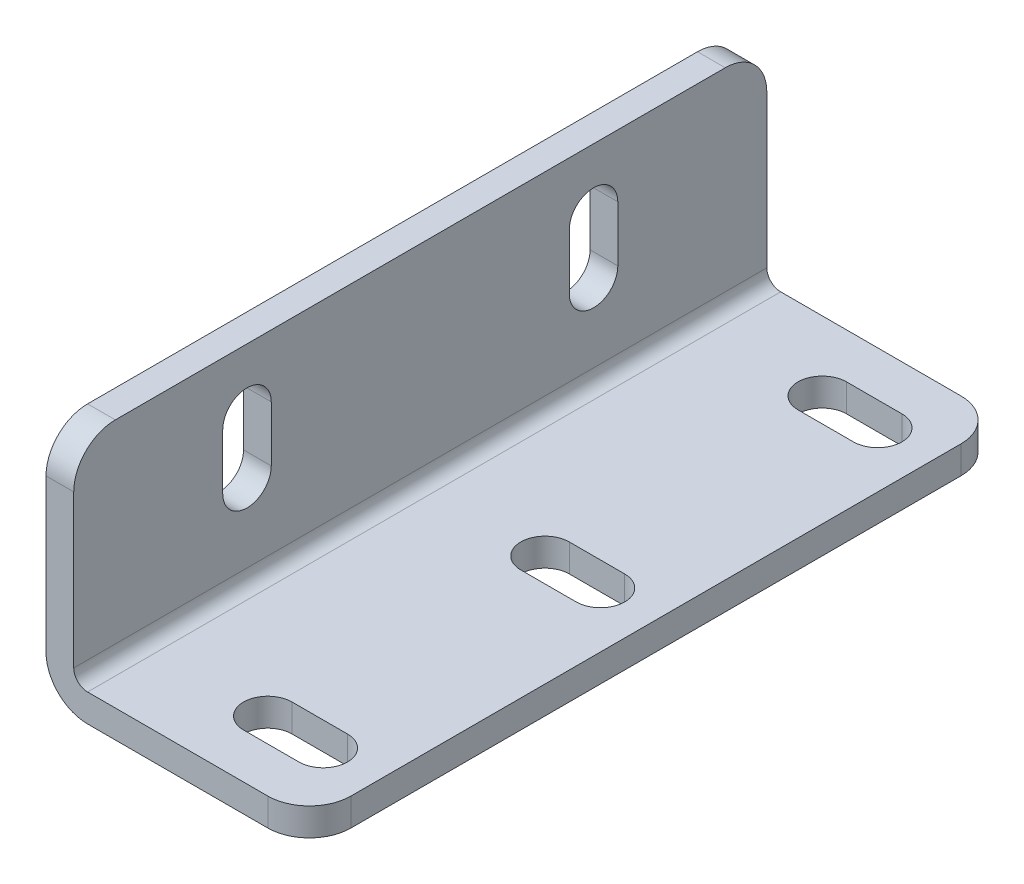
from build123d import *

# Parameters (mm, degrees)
EXTRUDE_1_DEPTH     = 25
CUT_EXTRUDE_1_DEPTH = 10
CUT_EXTRUDE_2_DEPTH = 10
FILLET_1_R          = 3
FILLET_2_R          = 1
FILLET_3_R          = 3


with BuildPart() as part:
    # 草图9 → 拉伸-薄壁1 (new, symmetric)
    with BuildSketch(Plane.XY):
        Polygon((17, 0), (0, 0), (0, 15), (-2, 15), (-2, -2), (17, -2), align=None)
    extrude(amount=EXTRUDE_1_DEPTH, both=True)

    # 草图10 → 切除-拉伸1 (cut)
    with BuildSketch(Plane(origin=(0, 0, 0), x_dir=(1, 0, 0), z_dir=(0, 1, 0))):
        with BuildLine():
            Line((9, 21.75), (13, 21.75))
            ThreePointArc((13, 21.75), (14.75, 20), (13, 18.25))
            Line((13, 18.25), (9, 18.25))
            ThreePointArc((9, 18.25), (7.25, 20), (9, 21.75))
        make_face()
        with BuildLine():
            Line((9, -21.75), (13, -21.75))
            ThreePointArc((13, -21.75), (14.75, -20), (13, -18.25))
            Line((13, -18.25), (9, -18.25))
            ThreePointArc((9, -18.25), (7.25, -20), (9, -21.75))
        make_face()
        with BuildLine():
            Line((9, 1.75), (13, 1.75))
            ThreePointArc((13, 1.75), (14.75, 0), (13, -1.75))
            Line((13, -1.75), (9, -1.75))
            ThreePointArc((9, -1.75), (7.25, 0), (9, 1.75))
        make_face()
    extrude(amount=-CUT_EXTRUDE_1_DEPTH, mode=Mode.SUBTRACT)

    # 草图11 → 切除-拉伸2 (cut)
    with BuildSketch(Plane(origin=(0, 0, 0), x_dir=(0, 0, -1), z_dir=(1, 0, 0))):
        with BuildLine():
            Line((-10.75, 10.5), (-10.75, 6.5))
            ThreePointArc((-10.75, 6.5), (-12.5, 4.75), (-14.25, 6.5))
            Line((-14.25, 6.5), (-14.25, 10.5))
            ThreePointArc((-14.25, 10.5), (-12.5, 12.25), (-10.75, 10.5))
        make_face()
        with BuildLine():
            Line((10.75, 10.5), (10.75, 6.5))
            ThreePointArc((10.75, 6.5), (12.5, 4.75), (14.25, 6.5))
            Line((14.25, 6.5), (14.25, 10.5))
            ThreePointArc((14.25, 10.5), (12.5, 12.25), (10.75, 10.5))
        make_face()
    extrude(amount=-CUT_EXTRUDE_2_DEPTH, mode=Mode.SUBTRACT)

    # 圆角1
    fillet_1_edges = [part.edges().sort_by_distance(p)[0] for p in [
        (-1, 15, 25),
        (-1, 15, -25),
        (17, -1, -25),
        (17, -1, 25),
    ]]
    fillet(fillet_1_edges, radius=FILLET_1_R)

    # 圆角2
    fillet_2_edges = [part.edges().sort_by_distance(p)[0] for p in [
        (0, 0, 0),
    ]]
    fillet(fillet_2_edges, radius=FILLET_2_R)

    # 圆角3
    fillet_3_edges = [part.edges().sort_by_distance(p)[0] for p in [
        (-2, -2, 0),
    ]]
    fillet(fillet_3_edges, radius=FILLET_3_R)


solid = part.part
